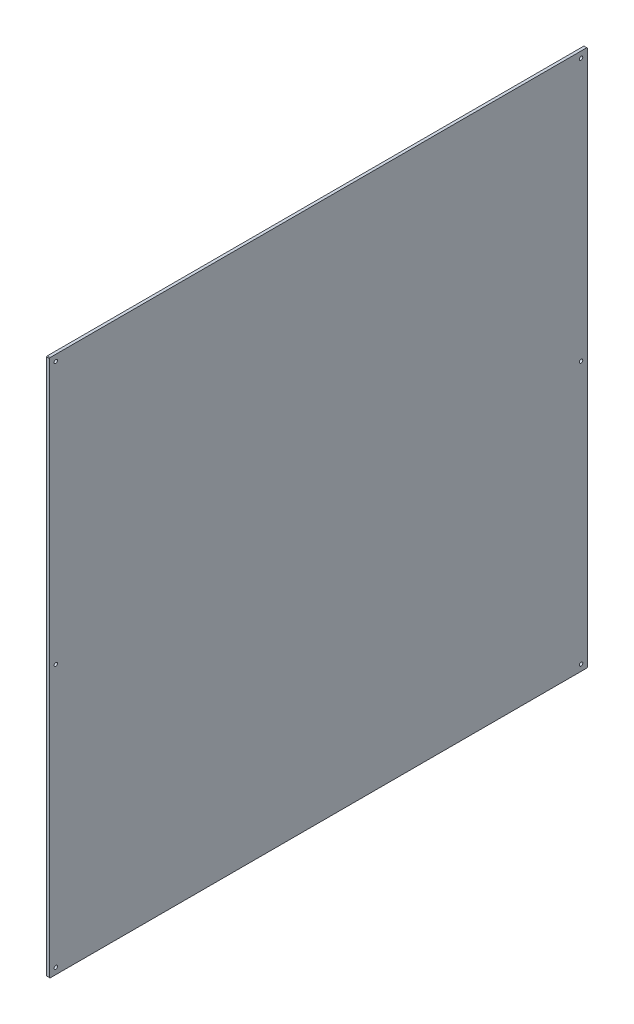
from build123d import *

# Parameters (mm, degrees)
SKETCH_1_W          = 938
SKETCH_1_H          = 937
EXTRUDE_1_DEPTH     = 5
CHAMFER_1_SIZE      = 1
SKETCH_2_R          = 3
CUT_EXTRUDE_1_DEPTH = 663.931557553


with BuildPart() as part:
    # 草图1 → 凸台-拉伸1 (new body)
    with BuildSketch(Plane(origin=(0, 0, 0), x_dir=(0, 0, -1), z_dir=(1, 0, 0))):
        Rectangle(SKETCH_1_W, SKETCH_1_H)
    extrude(amount=EXTRUDE_1_DEPTH)

    # 倒角1
    chamfer_1_edges = [part.edges().sort_by_distance(p)[0] for p in [
        (2.5, 468.5, 469),
        (2.5, 468.5, -469),
        (2.5, -468.5, -469),
        (2.5, -468.5, 469),
    ]]
    chamfer(chamfer_1_edges, length=CHAMFER_1_SIZE)

    # 草图2 → 切除-拉伸1 (cut, through all)
    with BuildSketch(Plane.ZY):
        with Locations((-458, 457.5)):
            Circle(SKETCH_2_R)
        with Locations(Location((-458, -457.5, 0), (0, 0, 180))):
            Circle(SKETCH_2_R)
        with Locations((458, -457.5)):
            Circle(SKETCH_2_R)
        with Locations(Location((458, 457.5, 0), (0, 0, 180))):
            Circle(SKETCH_2_R)
        with Locations((458, 0)):
            Circle(SKETCH_2_R)
        with Locations((-458, 0)):
            Circle(SKETCH_2_R)
    extrude(amount=-CUT_EXTRUDE_1_DEPTH, mode=Mode.SUBTRACT)


solid = part.part
